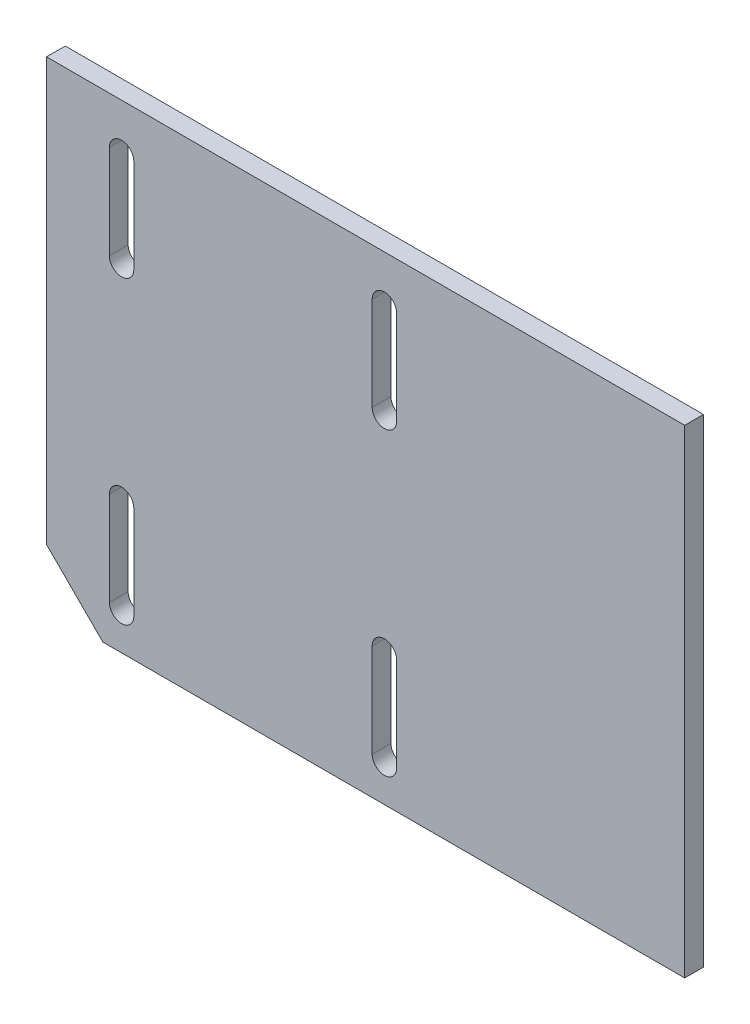
from build123d import *

# Parameters (mm, degrees)
BOSS_EXTRUDE1_DEPTH = 10


with BuildPart() as part:
    # Sketch1 → Boss-Extrude1 (new body)
    with BuildSketch(Plane.XY):
        Polygon((0, 0), (-340, 0), (-340, -225), (-310, -255), (0, -255), align=None)
        with BuildLine():
            Line((-293.5, -25), (-293.5, -75))
            ThreePointArc((-293.5, -75), (-300, -81.5), (-306.5, -75))
            Line((-306.5, -75), (-306.5, -25))
            ThreePointArc((-306.5, -25), (-300, -18.5), (-293.5, -25))
        make_face(mode=Mode.SUBTRACT)
        with BuildLine():
            Line((-153.5, -25), (-153.5, -75))
            ThreePointArc((-153.5, -75), (-160, -81.5), (-166.5, -75))
            Line((-166.5, -75), (-166.5, -25))
            ThreePointArc((-166.5, -25), (-160, -18.5), (-153.5, -25))
        make_face(mode=Mode.SUBTRACT)
        with BuildLine():
            Line((-293.5, -185), (-293.5, -235))
            ThreePointArc((-293.5, -235), (-300, -241.5), (-306.5, -235))
            Line((-306.5, -235), (-306.5, -185))
            ThreePointArc((-306.5, -185), (-300, -178.5), (-293.5, -185))
        make_face(mode=Mode.SUBTRACT)
        with BuildLine():
            Line((-153.5, -185), (-153.5, -235))
            ThreePointArc((-153.5, -235), (-160, -241.5), (-166.5, -235))
            Line((-166.5, -235), (-166.5, -185))
            ThreePointArc((-166.5, -185), (-160, -178.5), (-153.5, -185))
        make_face(mode=Mode.SUBTRACT)
    extrude(amount=-BOSS_EXTRUDE1_DEPTH)


solid = part.part
